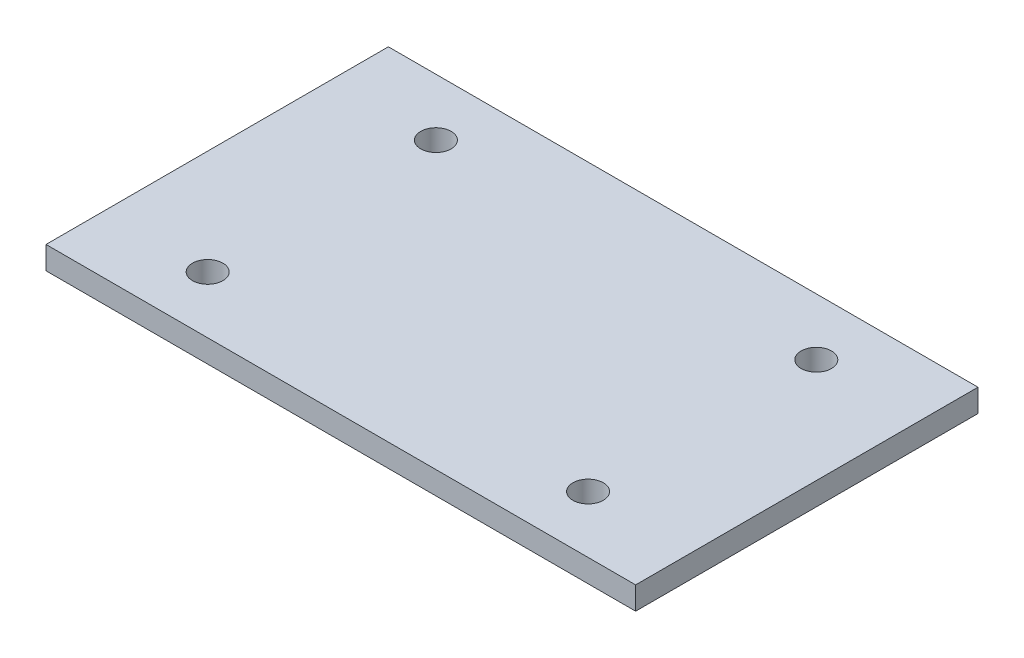
SolidWorks part; units mm, degrees
material "普通碳钢"
ref_plane "Front Plane" through (0, 0, 0) normal (0, 0, 1) x (1, 0, 0)
ref_plane "Top Plane" through (0, 0, 0) normal (0, 1, 0) x (1, 0, 0)
ref_plane "Right Plane" through (0, 0, 0) normal (1, 0, 0) x (0, 0, -1)
sketch "Sketch1" plane through (0, 0, 0) normal (0, 1, 0) x (1, 0, 0)
  line L0 (-100, 60) -> (100, 60) construction
  line L1 (-100, 60) -> (-100, -60) construction
  line L2 (-155, 90) -> (155, 90)
  line L3 (155, 90) -> (155, -90)
  line L4 (155, -90) -> (-155, -90)
  line L5 (-155, -90) -> (-155, 90)
  circle A0 centre (100, -60) radius 8
  circle A1 centre (-100, -60) radius 8
  circle A2 centre (-100, 60) radius 8
  circle A3 centre (100, 60) radius 8
  point P8 (0, 60)
  point P9 (-100, 0)
  dimension "D1" = 16
  dimension "D2" = 16
  dimension "D3" = 16
  dimension "D4" = 16
  dimension "D5" = 200
  dimension "D6" = 120
  dimension "D7" = 200
  dimension "D8" = 180
  dimension "D9" = 310
  dimension "D10" = 55
  dimension "D11" = 30
extrude "Extrude1" add sketch "Sketch1" along normal mid plane 12
